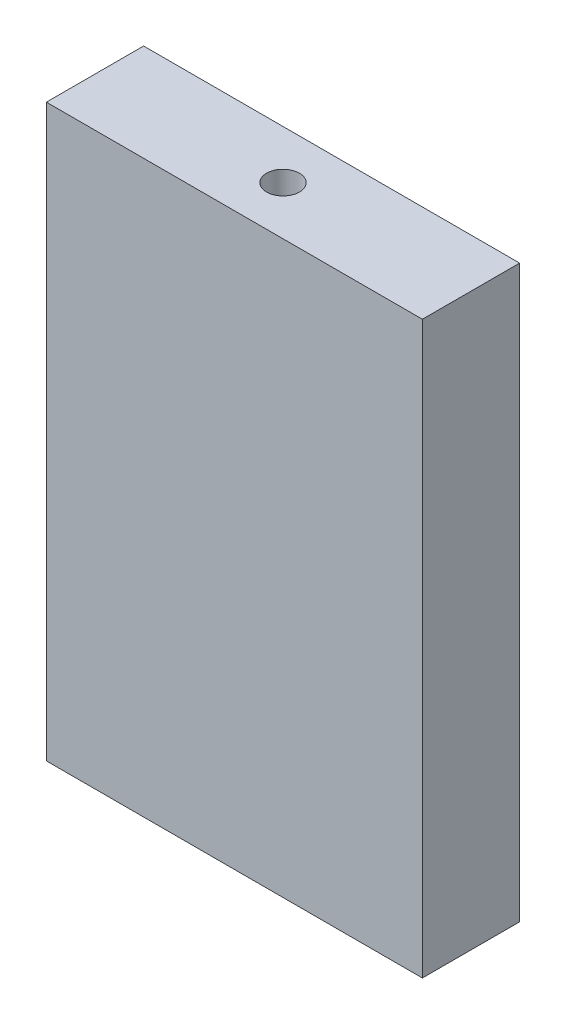
from build123d import *

# Parameters (mm, degrees)
SKETCH1_W           = 116
SKETCH1_H           = 176
BOSS_EXTRUDE1_DEPTH = 30
SKETCH3_R           = 5.055
CUT_EXTRUDE1_DEPTH  = 188.723200484


with BuildPart() as part:
    # Sketch1 → Boss-Extrude1 (new body)
    with BuildSketch(Plane.XY):
        Rectangle(SKETCH1_W, SKETCH1_H)
    extrude(amount=BOSS_EXTRUDE1_DEPTH)

    # Sketch3 → Cut-Extrude1 (cut, through all)
    with BuildSketch(Plane(origin=(0, 88, 0), x_dir=(1, 0, 0), z_dir=(0, 1, 0))):
        with Locations(Location((0, -15, 0), (0, 0, 180))):
            Circle(SKETCH3_R)
    extrude(amount=-CUT_EXTRUDE1_DEPTH, mode=Mode.SUBTRACT)


solid = part.part
